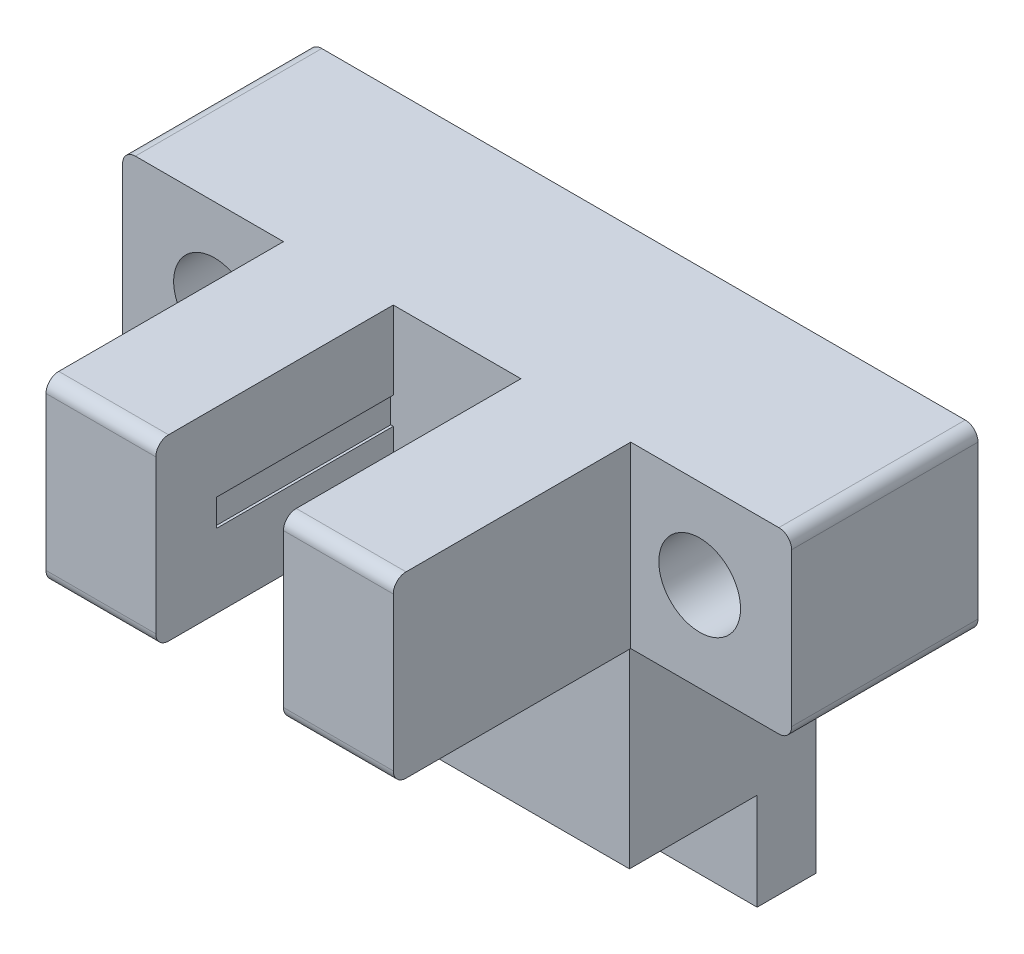
SolidWorks part; units mm, degrees
ref_plane "前视基准面" through (0, 0, 0) normal (0, 0, 1) x (1, 0, 0)
ref_plane "上视基准面" through (0, 0, 0) normal (0, 1, 0) x (1, 0, 0)
ref_plane "右视基准面" through (0, 0, 0) normal (1, 0, 0) x (0, 0, -1)
sketch "草图1" plane through (0, 0, 0) normal (0, 0, 1) x (1, 0, 0)
  line L1 (-13.1, 9.15) -> (13.1, 9.15)
  line L2 (-13.1, 9.15) -> (-13.1, -9.15)
  line L3 (-13.1, -9.15) -> (13.1, -9.15)
  line L4 (13.1, 9.15) -> (13.1, -9.15)
  line L5 (-13.1, 9.15) -> (13.1, -9.15) construction
  line L6 (-13.1, -9.15) -> (13.1, 9.15) construction
  point P0 (0, 0)
  dimension "D1" = 26.2
  dimension "D2" = 18.3
extrude "凸台-拉伸1" add sketch "草图1" along normal blind 7.3
sketch "草图2" plane through (0, 0, 7.3) normal (0, 0, 1) x (1, 0, 0)
  line L0 (0, 0) -> (0, 50000) construction
  line L1 (-13.1, 9.15) -> (-13.1, -9.15) construction
  line L2 (-13.1, 2.15) -> (-6.75, 2.15)
  line L3 (-13.1, 2.15) -> (-13.1, -9.15)
  line L4 (-13.1, -9.15) -> (-6.75, -9.15)
  line L5 (-6.75, 2.15) -> (-6.75, -9.15)
  line L6 (-13.1, -9.15) -> (13.1, -9.15) construction
  line L7 (6.75, 2.15) -> (6.75, -9.15)
  line L8 (13.1, -9.15) -> (6.75, -9.15)
  line L9 (13.1, 2.15) -> (13.1, -9.15)
  line L10 (13.1, 2.15) -> (6.75, 2.15)
  line L11 (13.1, 9.15) -> (-13.1, 9.15) construction
  dimension "D1" = 7
  dimension "D2" = 13.5
extrude "切除-拉伸1" cut sketch "草图2" against normal through all
sketch "草图3" plane through (0, 0, 7.3) normal (0, 0, 1) x (1, 0, 0)
  line L0 (0, 0) -> (0, 50000) construction
  line L1 (13.1, 9.15) -> (-13.1, 9.15) construction
  line L2 (-6.8, 9.15) -> (-2.5, 9.15)
  line L3 (-6.8, 9.15) -> (-6.8, 2.15)
  line L4 (-6.8, 2.15) -> (-2.5, 2.15)
  line L5 (-2.5, 9.15) -> (-2.5, 2.15)
  line L6 (2.5, 9.15) -> (2.5, 2.15)
  line L7 (6.8, 2.15) -> (2.5, 2.15)
  line L8 (6.8, 9.15) -> (6.8, 2.15)
  line L9 (6.8, 9.15) -> (2.5, 9.15)
  line L10 (13.1, 2.15) -> (6.75, 2.15) construction
  dimension "D1" = 5
  dimension "D2" = 4.3
extrude "凸台-拉伸2" add sketch "草图3" along normal blind 9.3
sketch "草图4" plane through (0, 0, 7.3) normal (0, 0, 1) x (1, 0, 0)
  line L0 (6.75, 2.15) -> (6.75, -9.15) construction
  line L1 (-6.75, -9.15) -> (6.75, -9.15)
  line L2 (-6.75, -9.15) -> (-6.75, -5.35)
  line L3 (-6.75, -5.35) -> (6.75, -5.35)
  line L4 (6.75, -9.15) -> (6.75, -5.35)
  dimension "D1" = 3.8
extrude "切除-拉伸2" cut sketch "草图4" against normal blind 5
sketch "草图5" plane through (0, 0, 7.3) normal (0, 0, 1) x (1, 0, 0)
  line L0 (-13.1, 5.65) -> (-50013.1, 5.65) construction
  line L1 (-13.1, 9.15) -> (-13.1, 2.15) construction
  line L2 (0, 0) -> (0, 50000) construction
  line L4 (-9.5, 5.65) -> (-9.5, 50005.65) construction
  circle A0 centre (-9.5, 5.65) radius 1.6
  circle A1 centre (9.5, 5.65) radius 1.6
  point P4 (-13.1, 5.65)
  dimension "D2" = 3.2
  dimension "D1" = 9.5
extrude "切除-拉伸3" cut sketch "草图5" against normal through all
sketch "草图6" plane through (-2.5, 0, 0) normal (1, 0, 0) x (0, 0, -1)
  line L0 (-7.3, 2.15) -> (-7.3, 9.15) construction
  line L1 (-14.2201, 6.0941) -> (-7.3, 6.0941)
  line L2 (-14.2201, 6.0941) -> (-14.2201, 5.0357)
  line L3 (-14.2201, 5.0357) -> (-7.3, 5.0357)
  line L4 (-7.3, 6.0941) -> (-7.3, 5.0357)
extrude "切除-拉伸4" cut sketch "草图6" against normal blind 0.1
fillet "圆角1" radius 0.5 4 edges at (13.1, 2.15, 3.65) (13.1, 9.15, 3.65) (-13.1, 2.15, 3.65) (-13.1, 9.15, 3.65)
mirror "镜向1" about plane through (0, 0, 0) normal (1, 0, 0) of "切除-拉伸4"
fillet "圆角2" radius 0.5 4 edges at (4.65, 2.15, 16.6) (4.65, 9.15, 16.6) (-4.65, 9.15, 16.6) (-4.65, 2.15, 16.6)
